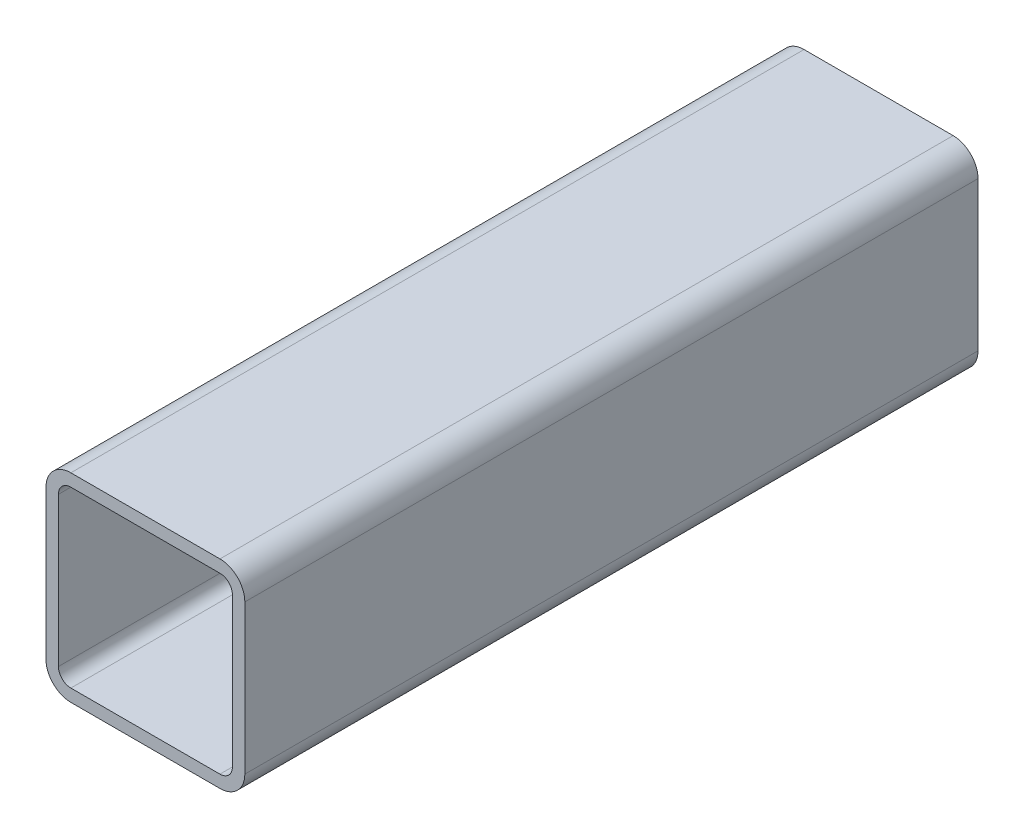
from build123d import *

# Parameters (mm, degrees)
BOSS_EXTRUDE_1_DEPTH = 118


with BuildPart() as part:
    # Sketch 1 → Boss-Extrude 1 (new, symmetric)
    with BuildSketch(Plane.XY):
        with BuildLine():
            Line((0, 32), (-24, 32))
            ThreePointArc((-24, 32), (-29.656854249, 29.656854249), (-32, 24))
            Line((-32, 24), (-32, 0))
            Line((-32, 0), (-32, -24))
            ThreePointArc((-32, -24), (-29.656854249, -29.656854249), (-24, -32))
            Line((-24, -32), (24, -32))
            ThreePointArc((24, -32), (29.656854249, -29.656854249), (32, -24))
            Line((32, -24), (32, 0))
            Line((32, 0), (32, 24))
            ThreePointArc((32, 24), (29.656854249, 29.656854249), (24, 32))
            Line((24, 32), (0, 32))
        make_face()
        with BuildLine():
            Line((0, 28), (-24, 28))
            ThreePointArc((-24, 28), (-26.828427125, 26.828427125), (-28, 24))
            Line((-28, 24), (-28, 0))
            Line((-28, 0), (-28, -24))
            ThreePointArc((-28, -24), (-26.828427125, -26.828427125), (-24, -28))
            Line((-24, -28), (24, -28))
            ThreePointArc((24, -28), (26.828427125, -26.828427125), (28, -24))
            Line((28, -24), (28, 0))
            Line((28, 0), (28, 24))
            ThreePointArc((28, 24), (26.828427125, 26.828427125), (24, 28))
            Line((24, 28), (0, 28))
        make_face(mode=Mode.SUBTRACT)
    extrude(amount=BOSS_EXTRUDE_1_DEPTH, both=True)


solid = part.part
